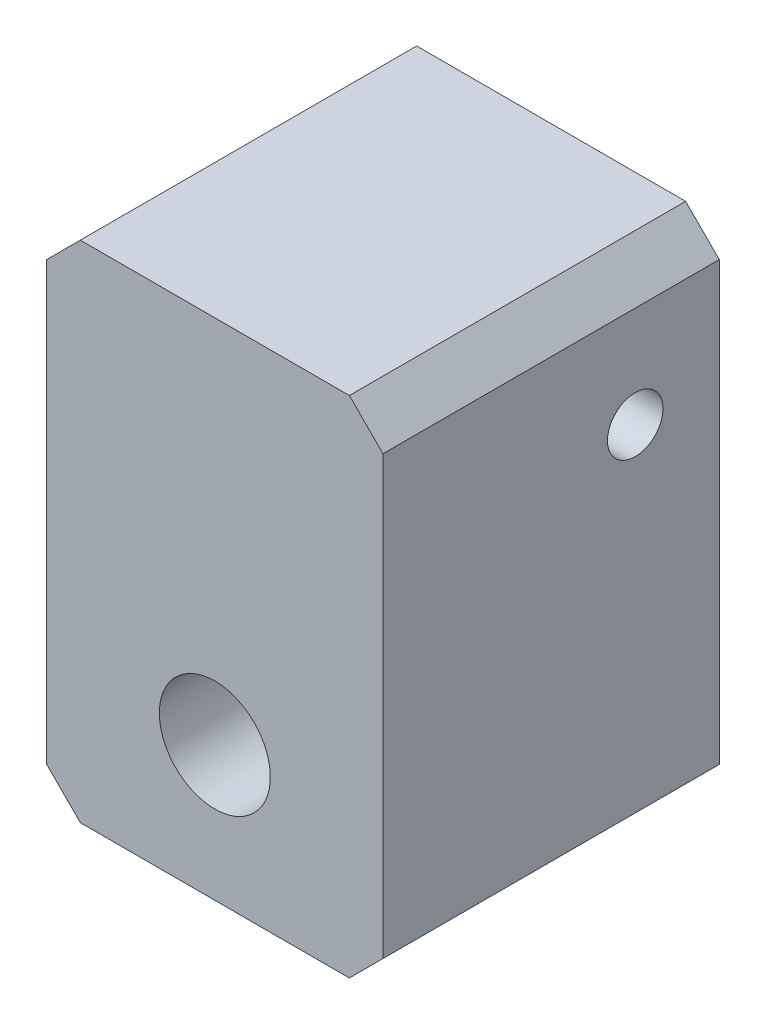
SolidWorks part; units mm, degrees
material "A6061"
ref_plane "前基準面" through (0, 0, 0) normal (0, 0, 1) x (1, 0, 0)
ref_plane "上基準面" through (0, 0, 0) normal (0, 1, 0) x (1, 0, 0)
ref_plane "右基準面" through (0, 0, 0) normal (1, 0, 0) x (0, 0, -1)
sketch "草图1" plane through (0, 0, 0) normal (0, 0, 1) x (1, 0, 0)
  line L1 (-10, 15) -> (10, 15)
  line L2 (-10, 15) -> (-10, -15)
  line L3 (-10, -15) -> (10, -15)
  line L4 (10, 15) -> (10, -15)
  line L5 (-10, 15) -> (10, -15) construction
  line L6 (-10, -15) -> (10, 15) construction
  point P0 (0, 0)
  dimension "D1" = 20
  dimension "D2" = 30
extrude "凸台-拉伸1" add sketch "草图1" along normal blind 20
hole_wizard "打孔尺寸根据内六角圆柱头螺钉的类型1" positions "草图3" profile "草图2" counterbore size "M6" standard "GB" end condition through all
sketch "草图3" plane through (3.1336, 10.9079, 0) normal (0, 0, 1) x (1, 0, 0)
  line L0 (-3.1336, -10.9079) -> (-3.1336, -25.1536) construction
  line L2 (-13.1336, -25.9079) -> (6.8664, -25.9079) construction
  point P0 (-3.1336, -17.9079)
  dimension "D1" = 8
sketch "草图2" plane through (0, -7, 0) normal (1, 0, 0) x (0, 1, 0)
  line L0 (0, 0) -> (0, 20)
  line L1 (0, 20) -> (3.3, 20)
  line L3 (3.3, 20) -> (3.3, 6.8)
  line L4 (3.3, 6.8) -> (5.5, 6.8)
  line L5 (5.5, 6.8) -> (5.5, 0)
  line L7 (5.5, 0) -> (0, 0)
  line L11 (0, -6.35) -> (0, 107.95) construction
  dimension "通孔孔直径" = 6.6
  dimension "通孔孔深度" = 20
  dimension "柱形沉头孔直径" = 11
  dimension "柱形沉头孔深度" = 6.8
hole_wizard "M4 螺纹孔1" positions "草图6" profile "草图5" tap size "M4" standard "GB" end condition through all
sketch "草图6" plane through (-10, 0, 0) normal (-1, 0, 0) x (0, 0, 1)
  line L4 (20, -15) -> (0, -15) construction
  line L5 (0, 15) -> (0, -15) construction
  point P0 (5, 7)
  dimension "D1" = 5
  dimension "D2" = 22
sketch "草图5" plane through (-10, 7, 5) normal (0, 1, 0) x (0, 0, 1)
  line L0 (0, 0) -> (0, 20)
  line L1 (0, 20) -> (1.65, 20)
  line L2 (1.65, 20) -> (1.65, 0)
  line L5 (1.65, 0) -> (0, 0)
  line L11 (0, -6.35) -> (0, 107.95) construction
  dimension "通孔螺纹孔钻头直径" = 3.3
  dimension "通孔螺纹孔钻头深度" = 20
cosmetic thread "孔螺蚊线1"
sketch "草图4" plane through (0, 0, 20) normal (0, 0, 1) x (1, 0, 0)
  line L0 (-10, -15) -> (10, -15) construction
  line L1 (-10, 15) -> (-7.5, 15)
  line L2 (-10, 15) -> (-10, 0)
  line L3 (-10, 0) -> (-7.5, 0)
  line L4 (-7.5, 15) -> (-7.5, 0)
  line L5 (10, 15) -> (-10, 15) construction
  line L6 (7.5, 0) -> (10, 0)
  line L7 (7.5, 0) -> (7.5, 15)
  line L8 (7.5, 15) -> (10, 15)
  line L9 (10, 0) -> (10, 15)
  line L10 (10, -15) -> (10, 15) construction
  line L11 (0, 0) -> (0, 9.4943) construction
  dimension "D1" = 15
  dimension "D2" = 15
chamfer "倒角1" distance 2 angle 45 4 edges at (-10, -15, 10) (-10, 15, 10) (10, 15, 10) (10, -15, 10)
